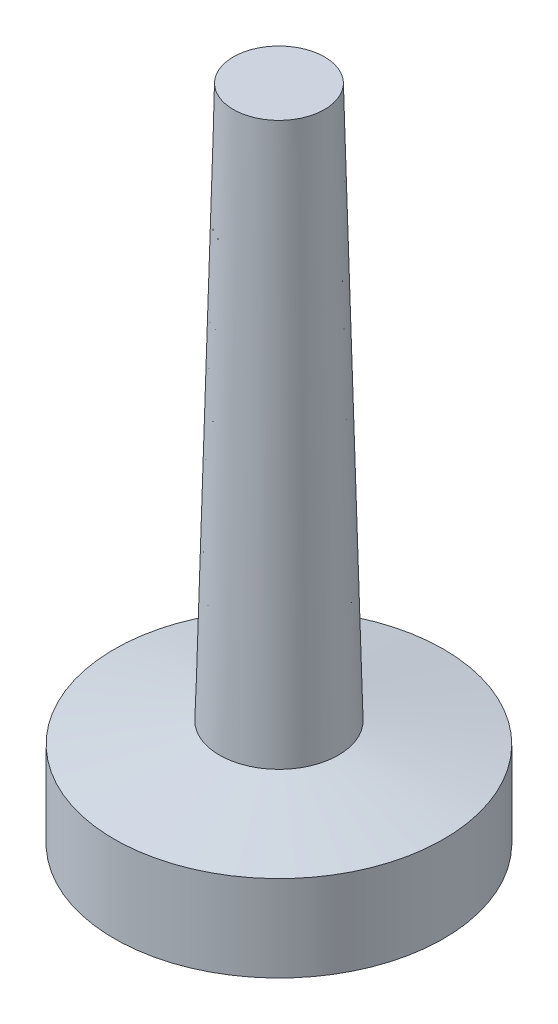
SolidWorks part; units mm, degrees
ref_plane "前视基准面" through (0, 0, 0) normal (0, 0, 1) x (1, 0, 0)
ref_plane "上视基准面" through (0, 0, 0) normal (0, 1, 0) x (1, 0, 0)
ref_plane "右视基准面" through (0, 0, 0) normal (1, 0, 0) x (0, 0, -1)
sketch "草图1" plane through (0, 0, 0) normal (1, 0, 0) x (0, 0, -1)
  line L27 (0, 0) -> (0, 130)
  line L30 (0, 130) -> (9, 130)
  line L31 (9, 130) -> (11.75, 21)
  line L46 (0, 0) -> (32.5, 0)
  line L47 (32.5, 17) -> (11.75, 21)
  line L48 (32.5, 17) -> (32.5, 0)
  dimension "D1" = 32.5
  dimension "D2" = 9
  dimension "D3" = 17
  dimension "D4" = 21
  dimension "D5" = 130
  dimension "D7" = 11.75
revolve "旋转1" add sketch "草图1" angle 360 about L27
sketch "草图2" plane through (0, 0, 0) normal (0, -1, 0) x (1, 0, 0)
  circle A0 centre (0, 0) radius 17.5
  dimension "D1" = 35
extrude "切除-拉伸1" cut sketch "草图2" against normal blind 10
sketch "草图3" plane through (0, 10, 0) normal (0, -1, 0) x (1, 0, 0)
  circle A0 centre (0, 0) radius 7.5
  dimension "D1" = 15
extrude "切除-拉伸2" cut sketch "草图3" against normal blind 10
